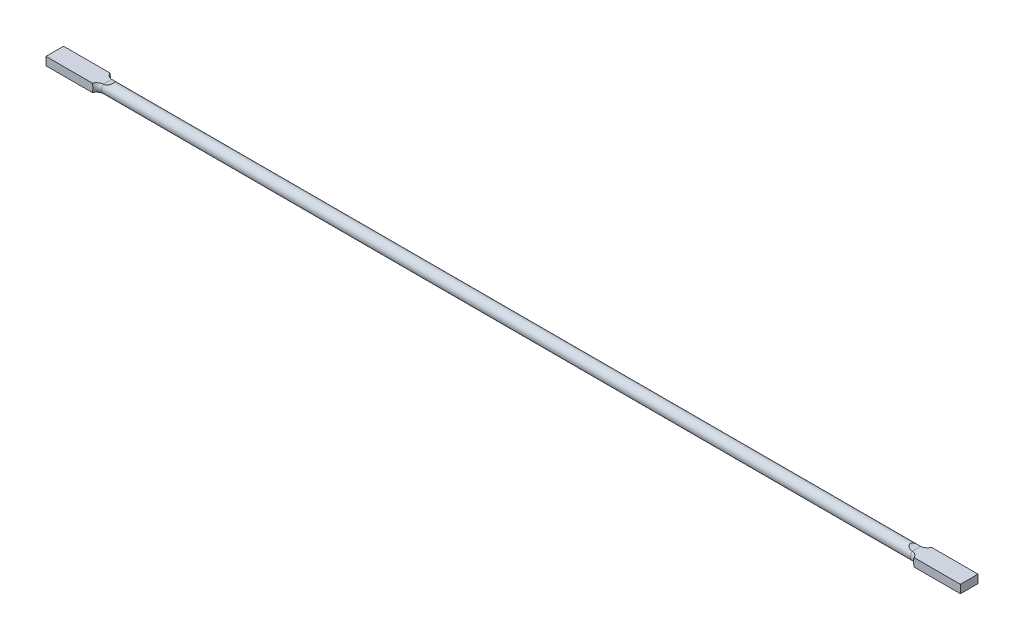
from build123d import *

# Parameters (mm, degrees)
SKETCH_1_W          = 45
SKETCH_1_H          = 15
EXTRUDE_1_DEPTH     = 3.5
CUT_EXTRUDE_1_DEPTH = 5
SKETCH_5_R          = 5
EXTRUDE_2_DEPTH     = 290


with BuildPart() as part:
    # 草图1 → 凸台-拉伸1 (new, symmetric)
    with BuildSketch(Plane(origin=(0, 0, 0), x_dir=(1, 0, 0), z_dir=(0, 1, 0))):
        with Locations((22.5, 0)):
            Rectangle(SKETCH_1_W, SKETCH_1_H)
    extrude(amount=EXTRUDE_1_DEPTH, both=True)

    # 草图2 → 旋转1 (revolve)
    with BuildSketch(Plane.XY, mode=Mode.PRIVATE) as revolve_1_sk:
        Polygon((45, 3.5), (45, 0), (100, 0), (100, 5), (50, 5), (45, 5), align=None)
    revolve(revolve_1_sk.sketch.rotate(Axis((3.468083249, 0, 0), (1, 0, 0)), 90), axis=Axis((3.468083249, 0, 0), (1, 0, 0)))

    # 草图3 → 切除-拉伸1 (cut, symmetric)
    with BuildSketch(Plane.XY):
        with BuildLine():
            Line((50, -5), (50, -7.872092098))
            Line((50, -7.872092098), (45, -7.872092098))
            Line((45, -7.872092098), (45, -3.5))
            ThreePointArc((45, -3.5), (47.610076627, -3.883077909), (50, -5))
        make_face()
        with BuildLine():
            Line((45, 3.5), (45, 6.877663773))
            Line((45, 6.877663773), (50, 6.877663773))
            Line((50, 6.877663773), (50, 5))
            ThreePointArc((50, 5), (47.610076627, 3.883077909), (45, 3.5))
        make_face()
    extrude(amount=CUT_EXTRUDE_1_DEPTH, both=True, mode=Mode.SUBTRACT)

    # 草图4 → 切除-旋转1 (revolve, cut)
    with BuildSketch(Plane(origin=(0, 0, 0), x_dir=(1, 0, 0), z_dir=(0, 1, 0))):
        with BuildLine():
            Line((40, 11.25), (45, 11.25))
            Line((45, 11.25), (45, 5))
            ThreePointArc((45, 5), (42.204915028, 5.659830056), (40, 7.5))
            ThreePointArc((40, 7.5), (39.341282089, 8.596434171), (38.919571519, 9.804009168))
            Line((38.919571519, 9.804009168), (40, 11.25))
        make_face()
    revolve(axis=Axis((45, 0, 0), (-1, 0, 0)), mode=Mode.SUBTRACT)

    # 草图5 → 凸台-拉伸2 (add)
    with BuildSketch(Plane(origin=(100, 0, 0), x_dir=(0, 0, -1), z_dir=(1, 0, 0))):
        with Locations(Location((0, 0, 0), (0, 0, 135.572995999))):
            Circle(SKETCH_5_R)
    extrude(amount=EXTRUDE_2_DEPTH)

    # 镜向1: part across plane


with BuildPart() as part_1:
    add(part.part)
    add(part.part.mirror(Plane(origin=(390, 0, 0), x_dir=(0, 0, 1), z_dir=(1, 0, 0))))


solid = part_1.part
